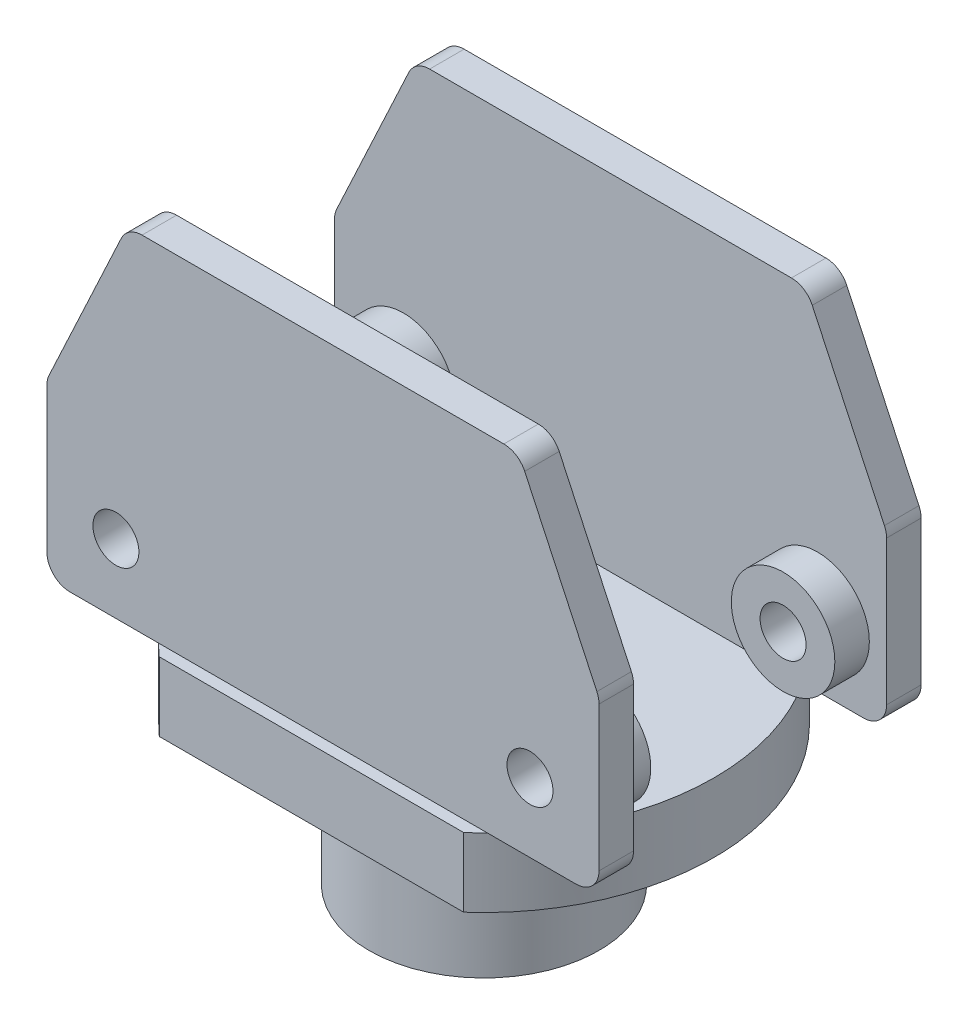
SolidWorks part; units mm, degrees
ref_plane "Front Plane" through (0, 0, 0) normal (0, 0, 1) x (1, 0, 0)
ref_plane "Top Plane" through (0, 0, 0) normal (0, 1, 0) x (1, 0, 0)
ref_plane "Right Plane" through (0, 0, 0) normal (1, 0, 0) x (0, 0, -1)
sketch "Sketch1" plane through (0, 0, 0) normal (0, 1, 0) x (1, 0, 0)
  circle A0 centre (0, 0) radius 50
  dimension "D1" = 100
extrude "Boss-Extrude1" add sketch "Sketch1" along normal blind 60
sketch "Sketch2" plane through (0, 60, 0) normal (0, 1, 0) x (1, 0, 0)
  circle A0 centre (0, 0) radius 100
  dimension "D1" = 200
extrude "Boss-Extrude2" add sketch "Sketch2" along normal blind 30
sketch "Sketch3" plane through (0, 60, 0) normal (0, -1, 0) x (1, 0, 0)
  line L0 (191.0183, 75) -> (5.8166, 170.5438)
  line L1 (-191.0183, -75) -> (191.0183, -75)
  line L3 (-191.0183, 75) -> (191.0183, 75)
  line L5 (-191.0183, -75) -> (191.0183, 75) construction
  line L6 (-191.0183, 75) -> (191.0183, -75) construction
  line L7 (5.8166, 170.5438) -> (-191.0183, 75)
  line L8 (191.0183, -75) -> (12.7966, -157.0492)
  line L9 (12.7966, -157.0492) -> (-191.0183, -75)
  point P0 (0, 0)
  dimension "D1" = 150
extrude "Cut-Extrude1" cut sketch "Sketch3" against normal through all
sketch "Sketch4" plane through (0, 90, 0) normal (0, 1, 0) x (1, 0, 0)
  line L0 (-66.1438, -75) -> (66.1438, -75) construction
  line L1 (-150, 70) -> (150, 70)
  line L2 (-150, 70) -> (-150, 55)
  line L3 (-150, 55) -> (150, 55)
  line L4 (150, 70) -> (150, 55)
  line L5 (-150, -55) -> (150, -55)
  line L6 (-150, -55) -> (-150, -70)
  line L7 (-150, -70) -> (150, -70)
  line L8 (150, -55) -> (150, -70)
  line L9 (66.1438, 75) -> (-66.1438, 75) construction
  point P11 (0, -75)
  dimension "D1" = 300
  dimension "D2" = 150
  dimension "D3" = 300
  dimension "D4" = 150
  dimension "D5" = 5
  dimension "D6" = 15
  dimension "D7" = 15
  dimension "D8" = 5
extrude "Boss-Extrude3" add sketch "Sketch4" along normal blind 150
sketch "Sketch5" plane through (0, 0, -70) normal (0, 0, -1) x (-1, 0, 0)
  line L0 (-150, 240) -> (150, 240) construction
  line L1 (-150, 90) -> (-120, 90)
  line L2 (-150, 90) -> (-150, 240)
  line L3 (-150, 240) -> (-120, 240)
  line L4 (-120, 90) -> (-120, 240)
  line L5 (71.4143, 90) -> (150, 90) construction
  line L6 (150, 90) -> (120, 90)
  line L7 (150, 90) -> (150, 240)
  line L8 (150, 240) -> (120, 240)
  line L9 (120, 90) -> (120, 240)
  line L10 (150, 240) -> (150, 90) construction
  dimension "D1" = 30
  dimension "D2" = 30
extrude "Cut-Extrude2" cut sketch "Sketch5" against normal through all
fillet "Fillet1" radius 10 8 edges at (-120, 240, 62.5) (120, 240, 62.5) (120, 240, -62.5) (-120, 240, -62.5) (120, 90, 62.5) (120, 90, -62.5) (-120, 90, 62.5) (-120, 90, -62.5)
sketch "Sketch6" plane through (0, 90, 0) normal (0, 1, 0) x (1, 0, 0)
  circle A0 centre (0, 0) radius 25
  dimension "D1" = 50
extrude "Cut-Extrude3" cut sketch "Sketch6" against normal blind 150
sketch "Sketch7" plane through (0, 0, -70) normal (0, 0, -1) x (-1, 0, 0)
  line L0 (71.4143, 90) -> (110, 90) construction
  line L1 (-110, 90) -> (-71.4143, 90) construction
  line L2 (-120, 100) -> (-120, 230) construction
  line L3 (120, 230) -> (120, 100) construction
  circle A0 centre (-90, 120) radius 10
  circle A1 centre (90, 120) radius 10
  dimension "D1" = 20
  dimension "D2" = 20
  dimension "D4" = 30
  dimension "D5" = 30
  dimension "D3" = 30
  dimension "D6" = 30
extrude "Cut-Extrude4" cut sketch "Sketch7" against normal through all
sketch "Sketch8" plane through (0, 0, 55) normal (0, 0, -1) x (-1, 0, 0)
  circle A0 centre (90, 120) radius 22.5
  circle A1 centre (-90, 120) radius 22.5
  circle A2 centre (-90, 120) radius 10
  circle A3 centre (90, 120) radius 10
  dimension "D1" = 45
  dimension "D2" = 45
extrude "Boss-Extrude4" add sketch "Sketch8" along normal blind 15 separate body
sketch "Sketch9" plane through (0, 0, -55) normal (0, 0, 1) x (1, 0, 0)
  circle A0 centre (90, 120) radius 10
  circle A1 centre (90, 120) radius 22.5
  circle A2 centre (-90, 120) radius 10
  circle A3 centre (-90, 120) radius 22.5
  dimension "D1" = 45
  dimension "D2" = 45
extrude "Boss-Extrude5" add sketch "Sketch9" along normal blind 15 separate body
sketch "Sketch10" plane through (0, 0, -70) normal (0, 0, -1) x (-1, 0, 0)
  line L0 (-120, 165) -> (-85, 240)
  line L1 (-120, 100) -> (-120, 230) construction
  line L2 (-110, 240) -> (110, 240) construction
  line L3 (120, 165) -> (85, 240)
  line L4 (120, 230) -> (120, 100) construction
  line L5 (-120, 165) -> (-120, 240)
  line L6 (-120, 240) -> (-85, 240)
  line L7 (120, 165) -> (120, 240)
  line L8 (120, 240) -> (85, 240)
  dimension "D1" = 35
  dimension "D2" = 35
extrude "Cut-Extrude5" cut sketch "Sketch10" against normal through all
fillet "Fillet2" radius 10 8 edges at (-85, 240, 62.5) (-120, 165, 62.5) (-120, 165, -62.5) (-85, 240, -62.5) (120, 165, 62.5) (120, 165, -62.5) (85, 240, -62.5) (85, 240, 62.5)
